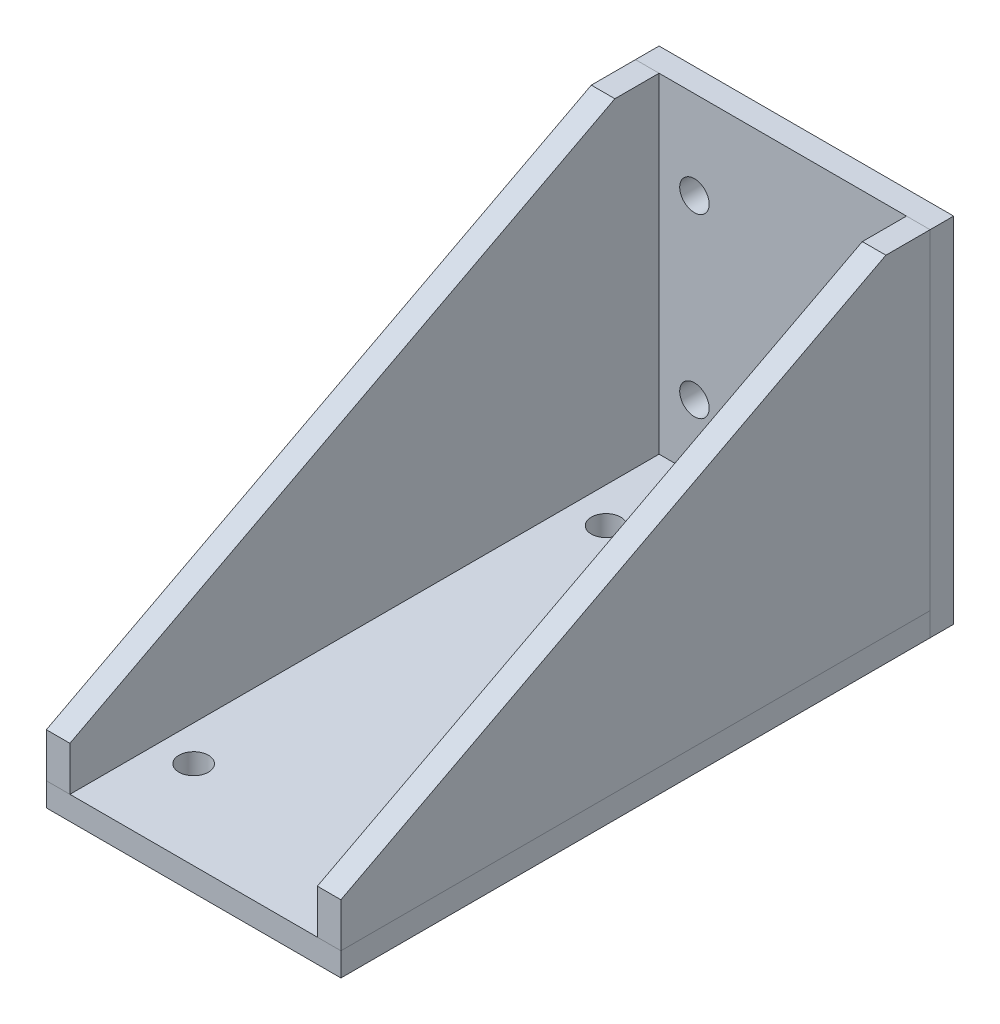
SolidWorks part; units mm, degrees
material "Q235"
ref_plane "Front Plane" through (0, 0, 0) normal (0, 0, 1) x (1, 0, 0)
ref_plane "Top Plane" through (0, 0, 0) normal (0, 1, 0) x (1, 0, 0)
ref_plane "Right Plane" through (0, 0, 0) normal (1, 0, 0) x (0, 0, -1)
sketch "Sketch1" plane through (0, 0, 0) normal (0, 0, 1) x (1, 0, 0)
  line L1 (-50, 60) -> (50, 60)
  line L2 (-50, 60) -> (-50, -60)
  line L3 (-50, -60) -> (50, -60)
  line L4 (50, 60) -> (50, -60)
  line L5 (-50, 60) -> (50, -60) construction
  line L6 (-50, -60) -> (50, 60) construction
  point P0 (0, 0)
  dimension "D1" = 100
  dimension "D2" = 120
extrude "Boss-Extrude1" add sketch "Sketch1" along normal blind 8
sketch "Sketch6" plane through (0, 0, 8) normal (0, 0, 1) x (1, 0, 0)
  line L0 (50, -60) -> (50, 60) construction
  line L1 (-50, -60) -> (50, -60)
  line L2 (-50, -60) -> (-50, -52)
  line L3 (-50, -52) -> (50, -52)
  line L4 (50, -60) -> (50, -52)
  dimension "D1" = 8
extrude "Boss-Extrude4" add sketch "Sketch6" along normal blind 200 separate body
sketch "Sketch3" plane through (-50, 0, 0) normal (-1, 0, 0) x (0, 0, 1)
  line L1 (208, -52) -> (208, -37)
  line L2 (208, -37) -> (23, 60)
  line L3 (23, 60) -> (8, 60)
  line L6 (8, 60) -> (8, -52)
  line L7 (8, -52) -> (208, -52)
  line L8 (8, 60) -> (8, -60) construction
  dimension "D1" = 15
  dimension "D2" = 200
  dimension "D3" = 15
extrude "Boss-Extrude2" add sketch "Sketch3" against normal blind 8 separate body
sketch "Sketch4" plane through (50, 0, 0) normal (1, 0, 0) x (0, 0, -1)
  line L5 (-8, -52) -> (-8, 60)
  line L6 (-208, -37) -> (-208, -52)
  line L7 (-23, 60) -> (-208, -37)
  line L8 (-8, 60) -> (-23, 60)
  line L9 (-8, -52) -> (-8, 60)
  line L11 (-208, -37) -> (-208, -52)
  line L12 (-23, 60) -> (-208, -37)
  line L13 (-8, 60) -> (-23, 60)
  line L15 (-208, -52) -> (-8, -52)
  line L16 (-208, -52) -> (-8, -52)
  dimension "D1" = 0
extrude "Boss-Extrude3" add sketch "Sketch4" against normal blind 8 separate body
hole_wizard "M8 Clearance Hole1" positions "Sketch7" profile "Sketch8" hole size "M8" standard "GB"
sketch "Sketch7" plane through (0, -52, 0) normal (0, 1, 0) x (1, 0, 0)
  line L0 (0, 0) -> (0, -37.4319) construction
  line L2 (50, -8) -> (-50, -8) construction
  point P0 (-30, -38)
  point P2 (30, -38)
  point P4 (-30, -178)
  point P6 (30, -178)
  dimension "D1" = 30
  dimension "D2" = 140
  dimension "D3" = 60
sketch "Sketch8" plane through (-30, -52, 38) normal (1, 0, 0) x (0, 0, 1)
  line L0 (0, 0) -> (0, 50.5043)
  line L1 (0, 50.5043) -> (5, 47.5)
  line L2 (5, 47.5) -> (5, 0)
  line L5 (5, 0) -> (0, 0)
  line L10 (0, 50.5043) -> (-5, 47.5) construction
  line L11 (0, -6.35) -> (0, 107.95) construction
  dimension "孔直径" = 10
  dimension "孔深度" = 47.5
  dimension "导头角度" = 118
hole_wizard "M8 Clearance Hole2" positions "Sketch10" profile "Sketch11" hole size "M8" standard "GB"
sketch "Sketch10" plane through (0, 0, 0) normal (0, 0, -1) x (-1, 0, 0)
  line L3 (-50, 60) -> (50, 60) construction
  line L4 (0, 60) -> (0, 45) construction
  point P0 (-30, 30)
  point P2 (30, 30)
  point P4 (30, -30)
  point P6 (-30, -30)
  dimension "D1" = 60
  dimension "D2" = 60
  dimension "D4" = 30
sketch "Sketch11" plane through (30, 30, 0) normal (1, 0, 0) x (0, 1, 0)
  line L0 (0, 0) -> (0, 50.5043)
  line L1 (0, 50.5043) -> (5, 47.5)
  line L2 (5, 47.5) -> (5, 0)
  line L5 (5, 0) -> (0, 0)
  line L10 (0, 50.5043) -> (-5, 47.5) construction
  line L11 (0, -6.35) -> (0, 107.95) construction
  dimension "孔直径" = 10
  dimension "孔深度" = 47.5
  dimension "导头角度" = 118
sketch "Sketch12" plane through (50, 0, 0) normal (1, 0, 0) x (0, 0, -1)
  line L0 (-208, -60) -> (-8, -60) construction
  line L1 (0, -60) -> (0, 60) construction
  circle A0 centre (-135, -25) radius 11
  dimension "D1" = 22
  dimension "D2" = 35
  dimension "D3" = 135
extrude "Cut-Extrude1" [suppressed] cut sketch "Sketch12" against normal through all
hole_wizard "M6 Tapped Hole2" positions "Sketch17" profile "Sketch18" tap size "M6" standard "GB"
sketch "Sketch17" [suppressed] plane through (50, 0, 0) normal (1, 0, 0) x (0, 0, -1)
  line L0 (-135, -30) -> (-135, -19) construction
  line L2 (-135, -30) -> (-111, -30) construction
  circle A0 centre (-135, -30) radius 11 construction
  point P0 (-159, -30)
  point P2 (-111, -30)
  dimension "D1" = 48
sketch "Sketch18" plane through (50, -30, 159) normal (0, 1, 0) x (0, 0, -1)
  line L0 (0, 0) -> (0, 100)
  line L1 (0, 100) -> (2.5, 100)
  line L2 (2.5, 100) -> (2.5, 0)
  line L5 (2.5, 0) -> (0, 0)
  line L11 (0, -6.35) -> (0, 107.95) construction
  dimension "通孔螺纹孔钻头直径" = 5
  dimension "通孔螺纹孔钻头深度" = 100
cosmetic thread "Cosmetic Thread2" parameters "D2"=6
cosmetic thread "Cosmetic Thread3" parameters "D2"=6
sketch "Sketch19" plane through (0, 0, 0) normal (0, 0, -1) x (-1, 0, 0)
  line L0 (-25, -37.5) -> (-25, -42.5) construction
  line L1 (-20, -37.5) -> (-20, -42.5)
  line L2 (-30, -37.5) -> (-30, -42.5)
  line L3 (0, 0) -> (0, -55.6605) construction
  line L4 (25, -37.5) -> (25, -42.5) construction
  line L5 (20, -37.5) -> (20, -42.5)
  line L6 (30, -37.5) -> (30, -42.5)
  line L7 (50, -60) -> (-50, -60) construction
  arc A0 (-20, -37.5) -> (-30, -37.5) centre (-25, -37.5) ccw
  arc A1 (-30, -42.5) -> (-20, -42.5) centre (-25, -42.5) ccw
  arc A2 (20, -37.5) -> (30, -37.5) centre (25, -37.5) cw
  arc A3 (30, -42.5) -> (20, -42.5) centre (25, -42.5) cw
  point P2 (-25, -40)
  point P12 (25, -40)
  dimension "D2" = 50
  dimension "D1" = 10
  dimension "D3" = 5
  dimension "D4" = 20
extrude "Cut-Extrude2" [suppressed] cut sketch "Sketch19" against normal blind 10
